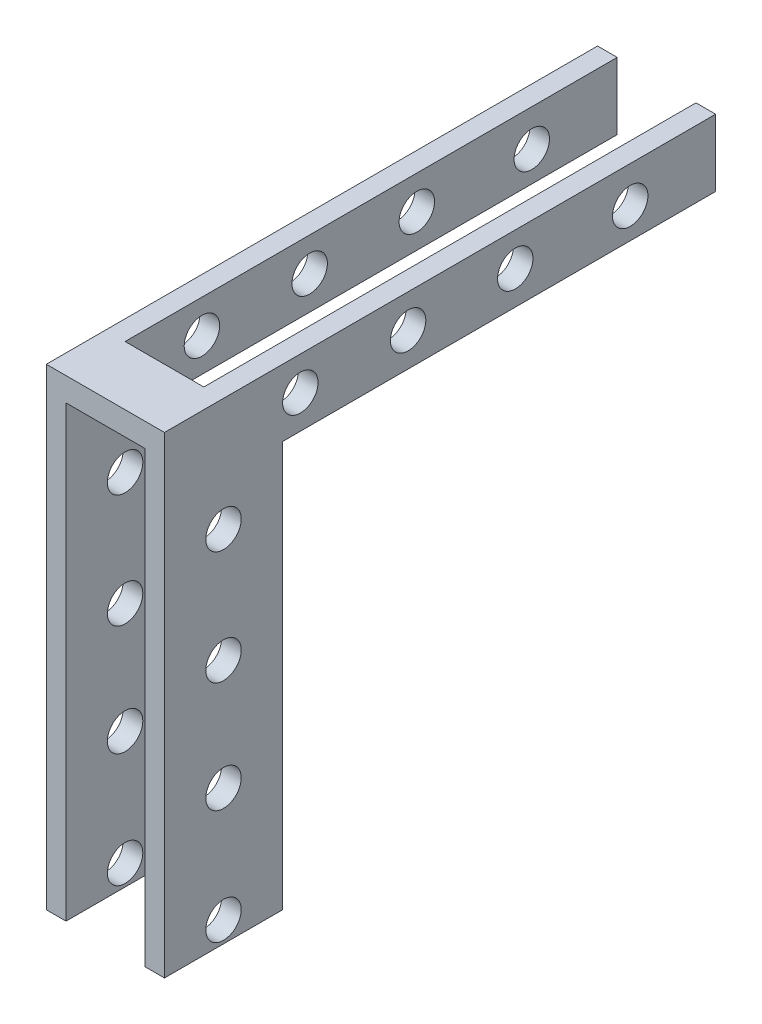
from build123d import *

# Parameters (mm, degrees)
SKETCH1_W             = 50
SKETCH1_H             = 300
BOSS_EXTRUDE1_DEPTH   = 1200
BOSS_EXTRUDE1_2_DEPTH = 1200
BOSS_EXTRUDE2_REACH   = 1236.909
SKETCH2_W             = 300
SKETCH2_H             = 60
SKETCH3_R             = 45
CUT_EXTRUDE1_DEPTH    = 900
SKETCH5_W             = 50
SKETCH5_H             = 170
BOSS_EXTRUDE3_DEPTH   = 900
SKETCH7_R             = 45
CUT_EXTRUDE2_DEPTH    = 900
SKETCH8_W             = 200
SKETCH8_H             = 150
CUT_EXTRUDE3_DEPTH    = 137
SKETCH9_R             = 45.000000002
CUT_EXTRUDE4_DEPTH    = 408
SKETCH10_R            = 45
CUT_EXTRUDE5_DEPTH    = 997
BOSS_EXTRUDE4_START   = -50
BOSS_EXTRUDE4_DEPTH   = 50
BOSS_EXTRUDE5_DEPTH   = 50


with BuildPart() as part:
    # Sketch1 → Boss-Extrude1 (new body)
    with BuildSketch(Plane(origin=(0, 0, 0), x_dir=(1, 0, 0), z_dir=(0, 1, 0))):
        with Locations((125, 0)):
            Rectangle(SKETCH1_W, SKETCH1_H)
    extrude(amount=BOSS_EXTRUDE1_DEPTH)

    # Sketch2 → Boss-Extrude2 (add, up to next)
    with BuildSketch(Plane(origin=(-100, 0, 0), x_dir=(0, 0, -1), z_dir=(1, 0, 0)), mode=Mode.PRIVATE) as boss_extrude2_sk1:
        with Locations((0, 1170)):
            Rectangle(SKETCH2_W, SKETCH2_H)
    boss_extrude2_tool1 = extrude(boss_extrude2_sk1.sketch, amount=BOSS_EXTRUDE2_REACH, mode=Mode.PRIVATE) - part.part


with BuildPart() as body_2:
    # Sketch1 → Boss-Extrude1 2 (new body)
    with BuildSketch(Plane(origin=(0, 0, 0), x_dir=(1, 0, 0), z_dir=(0, 1, 0))):
        with Locations((-125, 0)):
            Rectangle(SKETCH1_W, SKETCH1_H)
    extrude(amount=BOSS_EXTRUDE1_2_DEPTH)


with BuildPart() as part_1:
    add(part.part)

    add(body_2.part)  # Boss-Extrude2 merges body 2
    add(boss_extrude2_tool1.solids().sort_by_distance((-100, 1170, 0))[0])

    # Sketch3 → Cut-Extrude1 (cut)
    with BuildSketch(Plane(origin=(150, 0, 0), x_dir=(0, 0, -1), z_dir=(1, 0, 0))):
        with Locations((0, 624)):
            Circle(SKETCH3_R)
        with Locations((0, 343)):
            Circle(SKETCH3_R)
        with Locations((0, 53)):
            Circle(SKETCH3_R)
    extrude(amount=-CUT_EXTRUDE1_DEPTH, mode=Mode.SUBTRACT)

    # Sketch5 → Boss-Extrude3 (add)
    with BuildSketch(Plane(origin=(0, 0, -150), x_dir=(-1, 0, 0), z_dir=(0, 0, -1))):
        with Locations((-125, 1115)):
            Rectangle(SKETCH5_W, SKETCH5_H)
        with Locations((125, 1115)):
            Rectangle(SKETCH5_W, SKETCH5_H)
    extrude(amount=BOSS_EXTRUDE3_DEPTH)

    # Sketch7 → Cut-Extrude2 (cut)
    with BuildSketch(Plane(origin=(150, 0, 0), x_dir=(0, 0, -1), z_dir=(1, 0, 0))):
        with Locations((468.812102097, 1115)):
            Circle(SKETCH7_R)
        with Locations((741.013548247, 1115)):
            Circle(SKETCH7_R)
        with Locations((195.161471607, 1115)):
            Circle(SKETCH7_R)
    extrude(amount=-CUT_EXTRUDE2_DEPTH, mode=Mode.SUBTRACT)

    # Sketch8 → Cut-Extrude3 (cut)
    with BuildSketch(Plane(origin=(0, 1200, 0), x_dir=(1, 0, 0), z_dir=(0, 1, 0))):
        with Locations((0, 75)):
            Rectangle(SKETCH8_W, SKETCH8_H)
    extrude(amount=-CUT_EXTRUDE3_DEPTH, mode=Mode.SUBTRACT)

    # Sketch9 → Cut-Extrude4 (cut)
    with BuildSketch(Plane(origin=(150, 0, 0), x_dir=(0, 0, -1), z_dir=(1, 0, 0))):
        with Locations((1032.951729484, 1106.805056962)):
            Circle(SKETCH9_R)
    extrude(amount=-CUT_EXTRUDE4_DEPTH, mode=Mode.SUBTRACT)

    # Sketch10 → Cut-Extrude5 (cut)
    with BuildSketch(Plane.ZY.offset(150)):
        with Locations((0, 912.304081816)):
            Circle(SKETCH10_R)
    extrude(amount=-CUT_EXTRUDE5_DEPTH, mode=Mode.SUBTRACT)

    # Sketch12 → Boss-Extrude4 (add)
    with BuildSketch(Plane.ZY.offset(150).offset(BOSS_EXTRUDE4_START)):
        with BuildLine():
            Line((-1050, 1200), (-1250, 1200))
            Line((-1250, 1200), (-1250, 1030))
            Line((-1250, 1030), (-1050, 1030))
            Line((-1050, 1030), (-1050, 1065.159451282))
            ThreePointArc((-1050, 1065.159451282), (-1077.951729484, 1106.805056962), (-1050, 1148.450662641))
            Line((-1050, 1148.450662641), (-1050, 1200))
        make_face()
    extrude(amount=BOSS_EXTRUDE4_DEPTH)

    # Sketch13 → Boss-Extrude5 (add)
    with BuildSketch(Plane(origin=(150, 0, 0), x_dir=(0, 0, -1), z_dir=(1, 0, 0))):
        with BuildLine():
            Line((1250, 1200), (1050, 1200))
            Line((1050, 1200), (1050, 1148.450662641))
            ThreePointArc((1050, 1148.450662641), (1077.951729484, 1106.805056962), (1050, 1065.159451282))
            Line((1050, 1065.159451282), (1050, 1030))
            Line((1050, 1030), (1250, 1030))
            Line((1250, 1030), (1250, 1200))
        make_face()
    extrude(amount=-BOSS_EXTRUDE5_DEPTH)


solid = part_1.part
